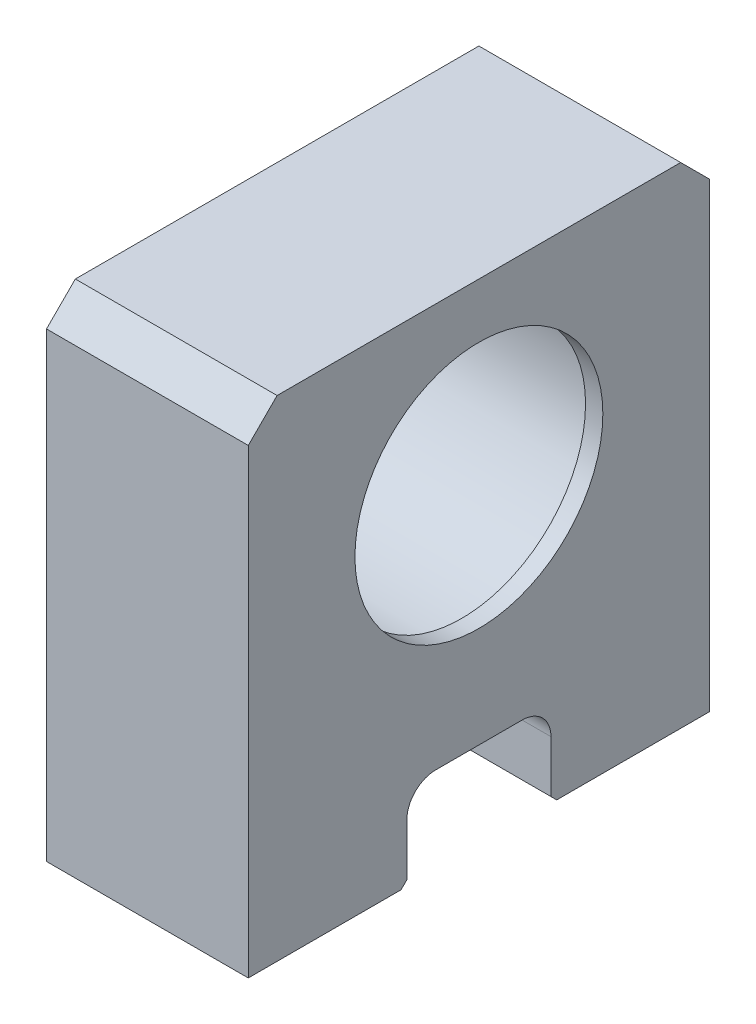
from build123d import *

# Parameters (mm, degrees)
SKETCH1_R             = 21.5
BOSS_EXTRUDE1_DEPTH   = 17.5
CHAMFER3_SIZE         = 5
FILLET1_R             = 5
M6_TAPPED_HOLE1_D     = 5
M6_TAPPED_HOLE1_DEPTH = 17
M6_TAPPED_HOLE1_TIP   = 1.502151548
SKETCH11_R            = 2.5
CUT_EXTRUDE1_DEPTH    = 15
CHAMFER4_SIZE         = 1
SKETCH12_R            = 26
CUT_EXTRUDE2_DEPTH    = 32
M4_TAPPED_HOLE1_D     = 3.3
M4_TAPPED_HOLE1_DEPTH = 11.5
M4_TAPPED_HOLE1_TIP   = 0.991420021
CHAMFER5_SIZE         = 0.5


with BuildPart() as part:
    # Sketch1 → Boss-Extrude1 (new, symmetric)
    with BuildSketch(Plane(origin=(0, 0, 0), x_dir=(0, 0, -1), z_dir=(1, 0, 0))):
        Polygon((-40, 85), (40, 85), (40, 0), (12.5, 0), (12.5, 15), (-12.5, 15), (-12.5, 0), (-40, 0), align=None)
        with Locations((0, 54)):
            Circle(SKETCH1_R, mode=Mode.SUBTRACT)
    extrude(amount=BOSS_EXTRUDE1_DEPTH, both=True)

    # Chamfer3
    chamfer3_edges = [part.edges().sort_by_distance(p)[0] for p in [
        (0, 85, 40),
        (0, 85, -40),
    ]]
    chamfer(chamfer3_edges, length=CHAMFER3_SIZE)

    # Fillet1
    fillet1_edges = [part.edges().sort_by_distance(p)[0] for p in [
        (0, 15, -12.5),
        (0, 15, 12.5),
    ]]
    fillet(fillet1_edges, radius=FILLET1_R)

    # M6 Tapped Hole1
    with Locations(Plane(origin=(0, 0, 0), x_dir=(-1, 0, 0), z_dir=(0, -1, 0))):
        with Locations((0, -32.5), (0, 32.5)):
            Hole(M6_TAPPED_HOLE1_D / 2, depth=M6_TAPPED_HOLE1_DEPTH)
            with Locations((0, 0, -(M6_TAPPED_HOLE1_DEPTH + M6_TAPPED_HOLE1_TIP / 2))):  # 118° drill point
                Cone(0, M6_TAPPED_HOLE1_D / 2, M6_TAPPED_HOLE1_TIP, mode=Mode.SUBTRACT)

    # Sketch11 → Cut-Extrude1 (cut)
    with BuildSketch(Plane.XZ):
        with Locations(Location((0, -20, 0), (0, 0, 270))):
            Circle(SKETCH11_R)
        with BuildLine():
            Line((2.5, 20.5), (2.5, 19.5))
            ThreePointArc((2.5, 19.5), (0, 17), (-2.5, 19.5))
            Line((-2.5, 19.5), (-2.5, 20.5))
            ThreePointArc((-2.5, 20.5), (0, 23), (2.5, 20.5))
        make_face()
    extrude(amount=-CUT_EXTRUDE1_DEPTH, mode=Mode.SUBTRACT)

    # Chamfer4
    chamfer4_edges = [part.edges().sort_by_distance(p)[0] for p in [
        (0, 0, -12.5),
        (0, 0, 12.5),
    ]]
    chamfer(chamfer4_edges, length=CHAMFER4_SIZE)

    # Sketch12 → Cut-Extrude2 (cut)
    with BuildSketch(Plane.ZY.offset(17.5)):
        with Locations((0, 54)):
            Circle(SKETCH12_R)
    extrude(amount=-CUT_EXTRUDE2_DEPTH, mode=Mode.SUBTRACT)

    # M4 Tapped Hole1
    with Locations(Plane.ZY.offset(17.5)):
        with Locations((-22.5, 74), (22.5, 74), (22.5, 34), (-22.5, 34)):
            Hole(M4_TAPPED_HOLE1_D / 2, depth=M4_TAPPED_HOLE1_DEPTH)
            with Locations((0, 0, -(M4_TAPPED_HOLE1_DEPTH + M4_TAPPED_HOLE1_TIP / 2))):  # 118° drill point
                Cone(0, M4_TAPPED_HOLE1_D / 2, M4_TAPPED_HOLE1_TIP, mode=Mode.SUBTRACT)

    # Chamfer5
    chamfer5_edges = [part.edges().sort_by_distance(p)[0] for p in [
        (-17.5, 54, -26),
    ]]
    chamfer(chamfer5_edges, length=CHAMFER5_SIZE)


solid = part.part
